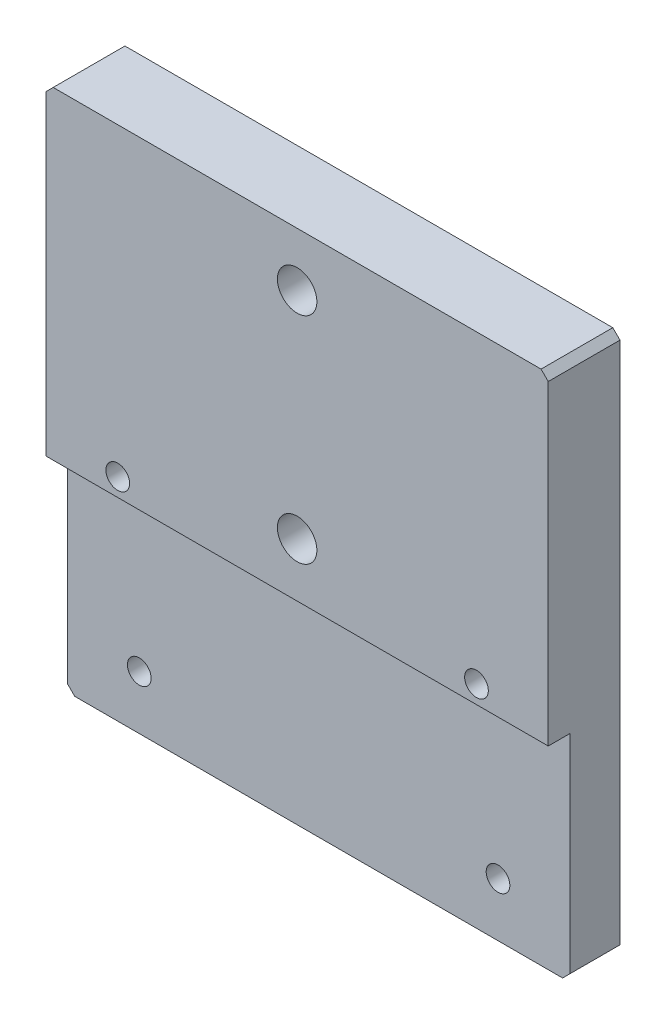
SolidWorks part; units mm, degrees
ref_plane "Front Plane" through (0, 0, 0) normal (0, 0, 1) x (1, 0, 0)
ref_plane "Top Plane" through (0, 0, 0) normal (0, 1, 0) x (1, 0, 0)
ref_plane "Right Plane" through (0, 0, 0) normal (1, 0, 0) x (0, 0, -1)
sketch "Sketch1" plane through (0, 0, 0) normal (0, 0, 1) x (1, 0, 0)
  line L1 (0, 0) -> (70, 0)
  line L2 (0, 0) -> (0, 75)
  line L3 (0, 75) -> (70, 75)
  line L4 (70, 0) -> (70, 75)
  dimension "D1" = 70
  dimension "D2" = 75
extrude "Boss-Extrude1" add sketch "Sketch1" along normal blind 10
sketch "Sketch2" plane through (0, 0, 0) normal (-1, 0, 0) x (0, 0, 1)
  line L1 (10, 0) -> (7, 0)
  line L2 (10, 0) -> (10, 30)
  line L3 (10, 30) -> (7, 30)
  line L4 (7, 0) -> (7, 30)
  dimension "D1" = 3
  dimension "D2" = 30
extrude "Cut-Extrude1" cut sketch "Sketch2" against normal through all
hole_wizard "M4 Tapped Hole1" positions "Sketch4" profile "Sketch3" tap size "M4" standard "GB"
sketch "Sketch4" plane through (0, 0, 0) normal (0, 0, -1) x (-1, 0, 0)
  point P0 (-10, 7.5)
  point P1 (-10, 32.5)
  point P4 (-60, 7.5)
  point P7 (-60, 32.5)
sketch "Sketch3" plane through (10, 7.5, 0) normal (1, 0, 0) x (0, 1, 0)
  line L0 (0, 0) -> (0, 12.4914)
  line L1 (0, 12.4914) -> (1.65, 11.5)
  line L2 (1.65, 11.5) -> (1.65, 0)
  line L5 (1.65, 0) -> (0, 0)
  line L10 (0, 12.4914) -> (-1.65, 11.5) construction
  line L11 (0, -6.35) -> (0, 107.95) construction
  dimension "螺纹孔钻头直径" = 3.3
  dimension "螺纹孔钻头深度" = 11.5
  dimension "导头角度" = 118
cosmetic thread "Cosmetic Thread1" parameters "D1"=8, "D2"=4
cosmetic thread "Cosmetic Thread2" parameters "D1"=7, "D2"=4
cosmetic thread "Cosmetic Thread3" parameters "D1"=8, "D2"=4
cosmetic thread "Cosmetic Thread4" parameters "D1"=7, "D2"=4
hole_wizard "Hole Size per Socket Head Cap Screw Type0" positions "Sketch6" profile "Sketch5" counterbore size "M5" standard "GB" end condition through all
sketch "Sketch6" plane through (0, 0, 0) normal (0, 0, -1) x (-1, 0, 0)
  line L4 (-35, 0) -> (-35, 75) construction
  line L5 (0, 0) -> (-70, 0) construction
  line L6 (-70, 75) -> (0, 75) construction
  line L8 (0, 37.5) -> (-70, 37.5) construction
  line L9 (0, 75) -> (0, 0) construction
  line L10 (-70, 0) -> (-70, 75) construction
  point P0 (-35, 37.5)
  point P1 (-35, 67.5)
  dimension "D1" = 30
  dimension "D2" = 7.5
sketch "Sketch5" plane through (35, 37.5, 0) normal (1, 0, 0) x (0, 1, 0)
  line L0 (0, 0) -> (0, 10)
  line L1 (0, 10) -> (2.75, 10)
  line L3 (2.75, 10) -> (2.75, 5.7)
  line L4 (2.75, 5.7) -> (5, 5.7)
  line L5 (5, 5.7) -> (5, 0)
  line L7 (5, 0) -> (0, 0)
  line L11 (0, -6.35) -> (0, 107.95) construction
  dimension "通孔孔直径" = 5.5
  dimension "通孔孔深度" = 10
  dimension "柱形沉头孔直径" = 10
  dimension "柱形沉头孔深度" = 5.7
chamfer "Chamfer1" distance 1 angle 45 4 edges at (70, 0, 3.5) (0, 0, 3.5) (0, 75, 5) (70, 75, 5)
